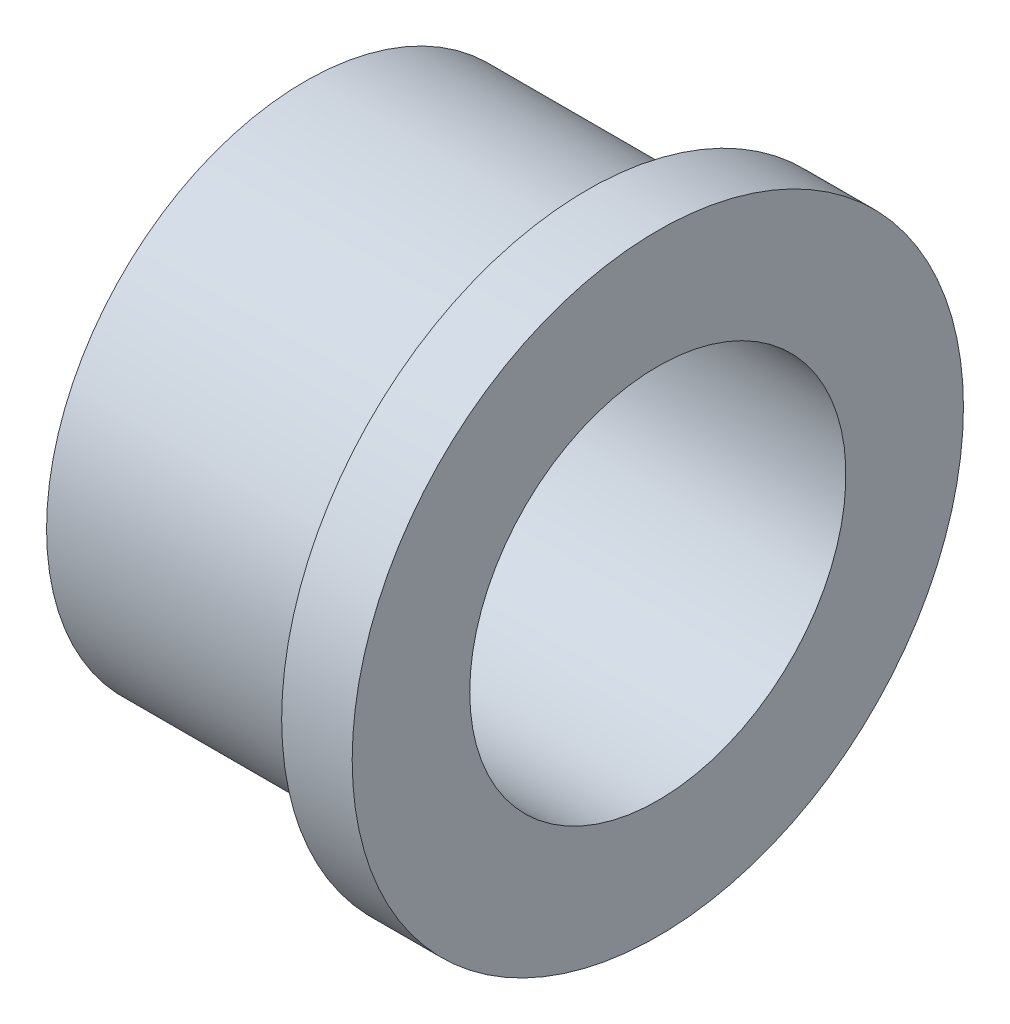
from build123d import *


with BuildPart() as part:
    # Sketch 1 → Revolve 1 (revolve)
    with BuildSketch(Plane.XY, mode=Mode.PRIVATE) as revolve_1_sk:
        Polygon((0, 32.5), (0, 20), (-37.5, 20), (-37.5, 27.5), (-7.5, 27.5), (-7.5, 32.5), align=None)
    revolve(revolve_1_sk.sketch.rotate(Axis((-54.785454848, 0, 0), (1, 0, 0)), 90), axis=Axis((-54.785454848, 0, 0), (1, 0, 0)))


solid = part.part
